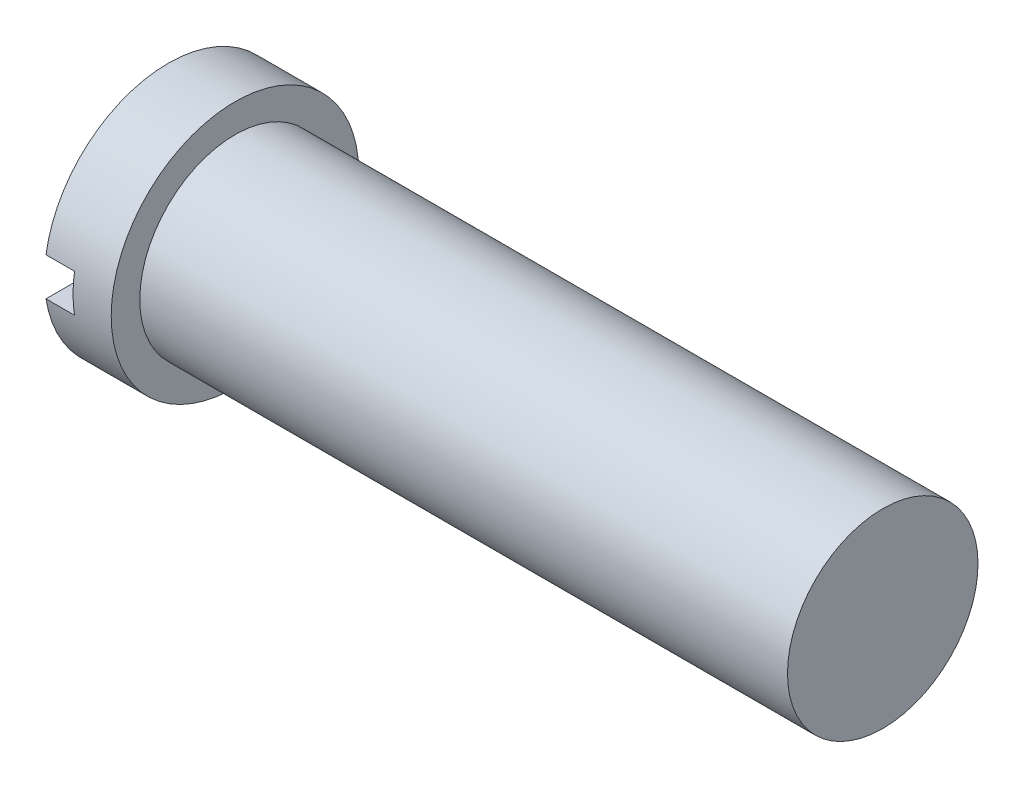
from build123d import *

# Parameters (mm, degrees)
CHAMFER_2_SIZE           = 1
CUT_EXTRUDE_1_DEPTH      = 49.38129804
CUT_EXTRUDE_1_DEPTH_BACK = 49.38129804
SKETCH_2_W               = 1.5
SKETCH_2_H               = 2
SKETCH_3_R               = 5.5
CUT_EXTRUDE_2_DEPTH      = 10


with BuildPart() as part:
    # 草图1 → 旋转1 (revolve)
    with BuildSketch(Plane.XY, mode=Mode.PRIVATE) as revolve_1_sk:
        Polygon((0, 0), (0, 6.5), (3.5, 6.5), (3.5, 5), (47.5, 5), (47.5, 0), align=None)
    revolve(revolve_1_sk.sketch.rotate(Axis((-19.421134541, 0, 0), (1, 0, 0)), 90), axis=Axis((-19.421134541, 0, 0), (1, 0, 0)))

    # 倒角2
    chamfer_2_edges = [part.edges().sort_by_distance(p)[0] for p in [
        (47.5, 0, -5),
    ]]
    chamfer(chamfer_2_edges, length=CHAMFER_2_SIZE)

    # 草图2 → 切除-拉伸1 (cut, two sides: drawn at the far end of the back side and taken through both)
    with BuildSketch(Plane.XY.offset(-CUT_EXTRUDE_1_DEPTH_BACK)):
        with Locations((0.75, 0)):
            Rectangle(SKETCH_2_W, SKETCH_2_H)
    extrude(amount=CUT_EXTRUDE_1_DEPTH + CUT_EXTRUDE_1_DEPTH_BACK, mode=Mode.SUBTRACT)

    # 草图3 → 切除-拉伸2 (cut)
    with BuildSketch(Plane(origin=(47.5, 0, 0), x_dir=(0, 0, -1), z_dir=(1, 0, 0))):
        Circle(SKETCH_3_R)
    extrude(amount=-CUT_EXTRUDE_2_DEPTH, mode=Mode.SUBTRACT)


solid = part.part
